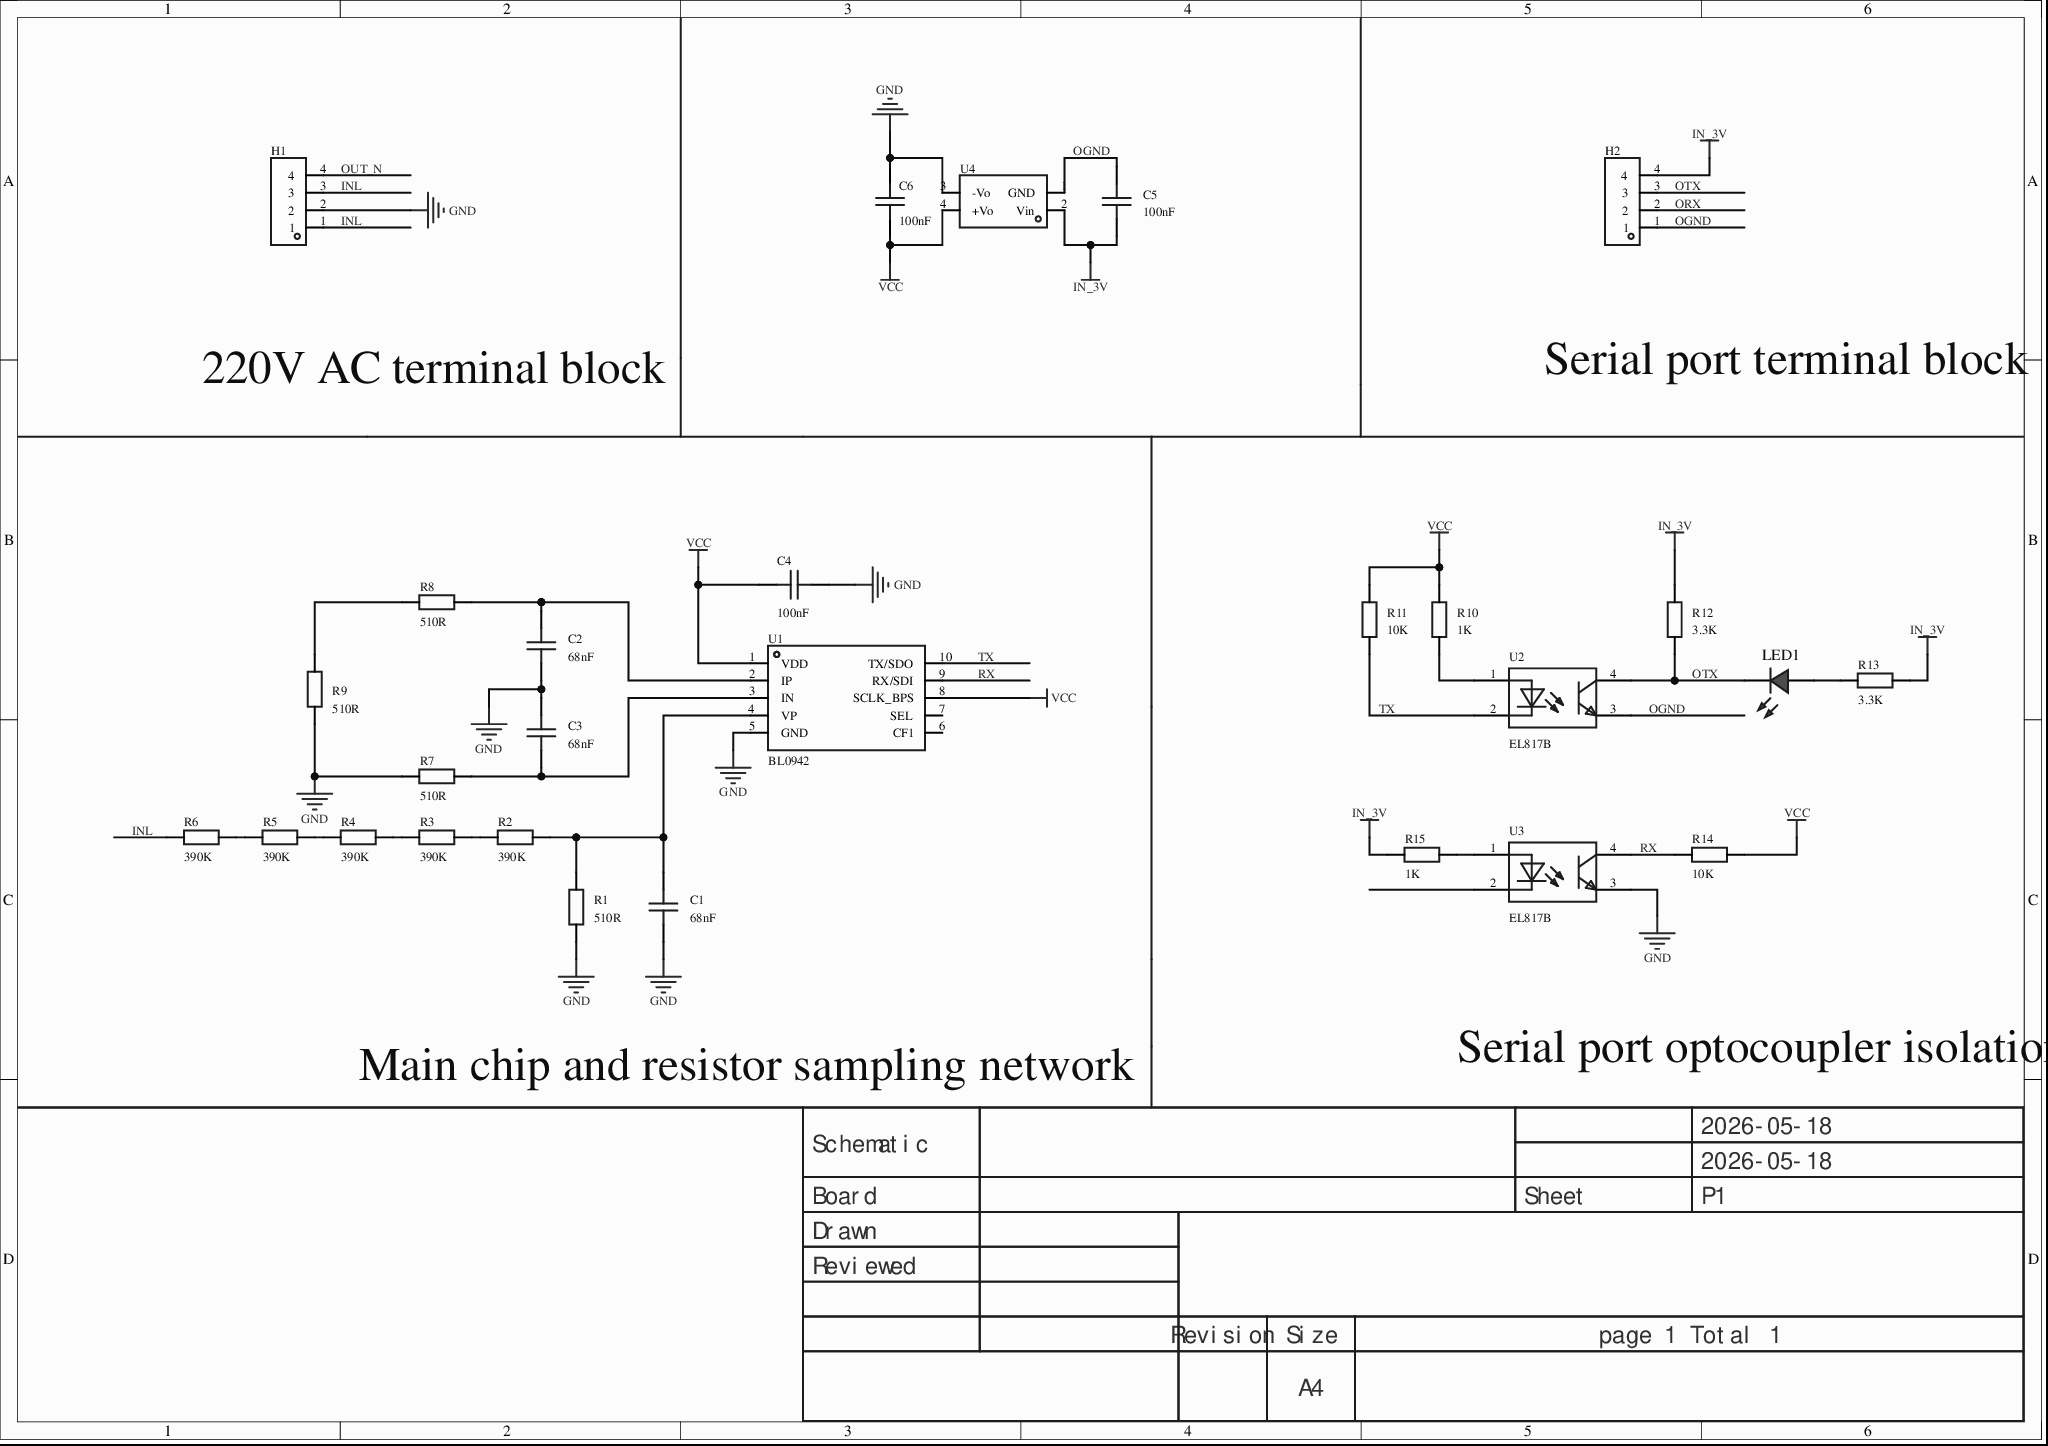
[diagram p0: MISC51247-3.schdoc]
# Altium project MISC51247-2.PrjPcb
1 sheet, 28 parts. Net scope: global (net labels, ports and power ports of the same name join across sheets).
Board file: MISC51247.pcbdoc

## Sheet MISC51247-3.schdoc
size 297 x 209 mm; Version: V1.0; @Project Name: MISC51247; @Update Date: 2026-05-18; @Create Date: 2026-05-18; @Board Name: MISC51247; @Create Time: 10:06:19; @Page Count: 1; @Page No: 1; @Schematic Name: MISC51247; @Update Time: 10:06:19; Size: A4

### Parts
C1  68nF  [C0603]
C2  68nF  [C0603]
C3  68nF  [C0603]
C4  100nF  [C0603]
C5  100nF  [C0603]
C6  100nF  [C0603]
H1  (no value)  [HDR-TH_4P-P2.54-V-F]
H2  (no value)  [HDR-TH_4P-P2.54-V-F]
LED1  (no value)  [LED_0603]
R1  510R  [R0603]
R2  390K  [R0603]
R3  390K  [R0603]
R4  390K  [R0603]
R5  390K  [R0603]
R6  390K  [R0603]
R7  510R  [R0603]
R8  510R  [R0603]
R9  510R  [R0603]
R10  1K  [R0603]
R11  10K  [R0603]
R12  3.3K  [R0603]
R13  3.3K  [R0603]
R14  10K  [R0603]
R15  1K  [R0603]
U1  BL0942  [SSOP-10_L4.9-W3.9-P1.00-LS6.0-BL]
U2  EL817B  [DIP-4_L6.5-W4.6-P2.54-LS7.6-BL]
U3  EL817B  [DIP-4_L6.5-W4.6-P2.54-LS7.6-BL]
U4  270kHz  [PWRM-TH_B0305S-1WR2]  (value not drawn)

### Nets
GND: C1.1 C2.1 C3.2 C4.1 C6.2 H1.2 R1.1 R7.2 R9.2 U1.5(GND) U3.3(EM) U4.3(-Vo)
IN_3V: C5.2 H2.4 R12.1 R13.2 R15.1 U4.2(Vin)
VCC: C4.2 C6.1 R10.1 R11.1 R14.2 U1.1(VDD) U1.8(SCLK_BPS) U4.4(+Vo)
INL: H1.1 H1.3 R6.2
OGND: C5.1 H2.1 U2.3(EM) U4.1(GND)
ORX: H2.2
OTX: H2.3 LED1.1(C) R12.2 U2.4(COL)
OUT_N: H1.4
RX: R14.1 U1.9(RX/SDI) U3.4(COL)
TX: R11.2 U1.10(TX/SDO) U2.2(CAT)
NetC1_2: C1.2 R1.2 R2.1 U1.4(VP)
NetC2_2: C2.2 R8.1 U1.2(IP)
NetC3_1: C3.1 R7.1 U1.3(IN)
NetLED1_2: LED1.2(A) R13.1
NetR2_2: R2.2 R3.1
NetR3_2: R3.2 R4.1
NetR4_2: R4.2 R5.1
NetR5_2: R5.2 R6.1
NetR8_2: R8.2 R9.1
NetR10_2: R10.2 U2.1(AN)
NetR15_2: R15.2 U3.1(AN)

Not connected (* = marked no-connect by the designer): U1 6(CF1)* 7(SEL)*; U3 2(CAT)

### Notes on the sheet
- 220V AC terminal block
- Serial port terminal block
- Main chip and resistor sampling network
- Serial port optocoupler isolation
- 2026-05-18
- Schematic
- Board
- Sheet
- P1
- Drawn
- Reviewed
- Revision
- Size
- A4
- page 1 Total 1

### Library data of the parts
C1-C6 = CAP_0603: Symbol: Capacitance; ConvertToPcb: yes; ModelId: ac125912035d415993ca9572d50418b10819f05c4eef4c71ace90d822a990e87; ModelName: C0603_L1.6-W0.8-H0.8; ModelTransform: 62.992,31.496,0,0,0,0,0,0,0; Device: CAP_0603; AddInBom: yes; Supplier Footprint: 0603; FootprintName: C0603
  C1-C3: Value: 68nF
  C4-C6: Value: 100nF
H1 H2 = HDR-F_2.54_1x4P: Symbol: 2.54-1*4P female; ConvertToPcb: yes; ModelId: d187812051054f85879fcaa51a310d8e0819f05c4eef4c71ace90d822a990e87; ModelTransform: 419.6842,98.464,0,0,0,0,0,0,-118.11; Device: HDR-F_2.54_1x4P; AddInBom: yes; SupplierPart: C2718488; Supplier Footprint: 插件; FootprintName: HDR-TH_4P-P2.54-V-F; ModelName: HDR-TH_4P-P2.54-V-F
LED1 = LED_0603-R: Symbol: LED_R; Convert to PCB: yes; 3D Model: dd8257b0d61a4cd7b68939a056e080950819f05c4eef4c71ace90d822a990e87; 3D Model Transform: 58.72,29.4,22.03,0,0,0,0,0,0; ModelName: LED-0603_R; Device: LED_0603-R; Add into BOM: yes; Supplier Footprint: 0603; FootprintName: LED_0603
R1-R15 = Res_0603: Symbol: Resistor; ConvertToPcb: yes; ModelId: fc143cca1e79419f9cd78b61e9279f080819f05c4eef4c71ace90d822a990e87; ModelTransform: 31.8897,63.7794,0,90,0,0,0,0,0; Device: Res_0603; AddInBom: yes; Supplier Footprint: 0603; FootprintName: R0603; ModelName: R0603
  R1 R7-R9: Value: 510R
  R2-R6: Value: 390K
  R10 R15: Value: 1K
  R11 R14: Value: 10K
  R12 R13: Value: 3.3K
U1 = BL0942_C2837510: BL0942 is an energy metering chip with built-in clock and no calibration needed, for single-phase multifunction meters, smart sockets, smart appliances and similar uses, with high cost performance.; Manufacturer: BL(上海贝岭); AddInBom: yes; ModelId: d633480e87ce4338a1764e9c79a3c6ca0819f05c4eef4c71ace90d822a990e87; ModelName: SSOP-10_L4.9-W3.9-H1.5-LS6.0-P1.00; ModelTransform: 228.57954,188.976,0,90,0,0,0,0,0; Symbol: BL0942; Device: BL0942_C2837510; LCSC Part Name: BL0942内置时钟免校准计量芯片; SupplierPart: C2837510; ManufacturerPart: BL0942; Supplier Footprint: SSOP-10-150mil; JLCPCB Part Class: Extended Part; Datasheet: https://atta.szlcsc.com/upload/public/pdf/source/20220627/BFAD44701CA6DE9A8853C5A4834B6884.pdf; Supplier: LCSC; ConvertToPcb: yes; FootprintName: SSOP-10_L4.9-W3.9-P1.00-LS6.0-BL
U2 U3 = EL817B: 输入类型:DC;正向压降(Vf):1.2V;输出电流:50mA;隔离电压(Vrms):5kV;直流反向耐压(Vr):6V;负载电压:80V;输出通道数:1;集射极饱和电压(VCE(sat)):100mV@20mA,1mA;; Manufacturer: AOTE(奥特); AddInBom: yes; ModelId: 2280cb24a5a64e61a6c27f1690450eca0819f05c4eef4c71ace90d822a990e87; ModelName: DIP-4_L6.5-W4.6-H3.5-LS7.62-P2.54; ModelTransform: 180.3146,311.8104,0,0,0,0,0.004,-0.002,-137.795; Input type: DC; Output Type: Phototransistor; Voltage - Forward(Vf): 1.2V; Output Current: 50mA; Isolation Voltage(Vrms): 5kV; Reverse Voltage: 6V; Load Voltage: 80V; Number of Outputs: 1; Rise time: 4us@2mA,100Ω; Fall time: 3us; Current Transfer Ratio (CTR) Minimum: 130%; Current Transfer Ratio (CTR) Maximum/Saturation Value: 260%; Symbol: EL817B; Device: EL817B; LCSC Part Name: 光耦-光电晶体管输出; SupplierPart: C42371501; ManufacturerPart: EL817B; Supplier Footprint: DIP-4; Datasheet: https://item.szlcsc.com/datasheet/EL817B/44252197.html; Supplier: LCSC; ConvertToPcb: yes; FootprintName: DIP-4_L6.5-W4.6-P2.54-LS7.6-BL; Vce Saturation(VCE(sat)): 100mV@20mA,1mA; Operating Temperature: -55℃~+110℃; Total Power Dissipation(Pd): -; Forward Current(If): 50mA
U4 = B0305S-1WR2: B0305S-1WR2是为客户提供小体积，高效率的微小功率，定电压，输入隔离非稳压，单路输出DC/DC模块电源；该系列产品是专门针对板上电源系统中需要产生一组与输入电源隔离的电压的应用场合而设计的。该产品适用于：输入电源的电压比较稳定（电压变化范围±10%Vin）;●输入输出之间要求隔离（隔离电压≤1500VDC）；●对输出电压稳定度要求不高；●典型应用：纯数字电路场合，一般低频模拟电路场合，继电器驱动电路，数据交换电路场合等.; Manufacturer: YLPTEC(易川); Symbol: B0305S-1WR2_C3031177; AddInBom: yes; Number of Channels: 1; Output Power: 1W; Voltage - Supply: 2.97V~3.63V; Conversion Efficiency: 76%; Output Voltage: 5V; Output Current(Max): 200mA; Capacitive Load(Max): 220uF; Isolation Voltage(Vrms): 1.5kV; No-Load Input Current: 13mA; Ripple Noise: 30mVp-p; Device: B0305S-1WR2; LCSC Part Name: 1W 隔离式 DC-DC 转换器; SupplierPart: C3031177; ManufacturerPart: B0305S-1WR2; Supplier Footprint: SIP,11.6x6mm; JLCPCB Part Class: Extended Part; Datasheet: https://item.szlcsc.com/datasheet/B0305S-1WR2/3567758.html; Supplier: LCSC; ConvertToPcb: yes; FootprintName: PWRM-TH_B0305S-1WR2; Type: Boost type; Features: Short-circuit protection; Operating Temperature: -40℃~+105℃; Value: 270kHz; Length: 11.6mm; Width: 6mm; Height: 10.16mm